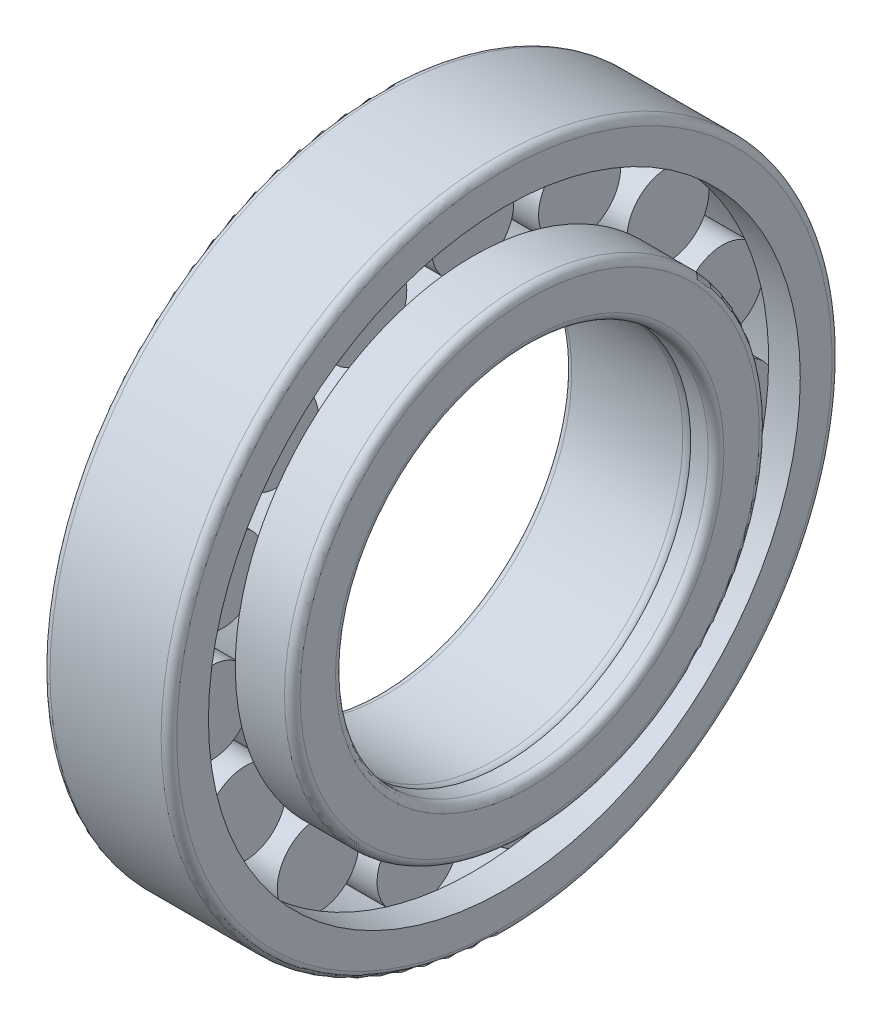
from build123d import *

# Parameters (mm, degrees)
SKETCH_3_W               = 17
SKETCH_3_H               = 11.0001
PATTERN_CIRCULAR_1_COUNT = 15


with BuildPart() as part:
    # 草图2 → Revolve 794 (revolve)
    with BuildSketch(Plane.XY, mode=Mode.PRIVATE) as revolve_794_sk:
        with BuildLine():
            Line((8.5, 59.5), (25.5, 59.5))
            Line((25.5, 59.5), (34, 57.222431864))
            Line((34, 57.222431864), (34, 52.1))
            ThreePointArc((34, 52.1), (33.38492424, 50.61507576), (31.9, 50))
            Line((31.9, 50), (2.1, 50))
            ThreePointArc((2.1, 50), (0.61507576, 50.61507576), (0, 52.1))
            Line((0, 52.1), (0, 63.7))
            Line((0, 63.7), (8.5, 63.7))
            Line((8.5, 63.7), (8.5, 59.5))
        make_face()
    revolve(revolve_794_sk.sketch.rotate(Axis((-10.080094127, 0, 0), (1, 0, 0)), 90), axis=Axis((-10.080094127, 0, 0), (1, 0, 0)))

    # 草图3 → 凸台-旋转1 (revolve)
    with BuildSketch(Plane.XY):
        with Locations((17, 64.99995)):
            Rectangle(SKETCH_3_W, SKETCH_3_H)
    revolve_1 = revolve(axis=Axis((-1.603948851, 70.5, 0), (1, 0, 0)))

    # 草图4 → 凸台-旋转2 (revolve)
    with BuildSketch(Plane.XY, mode=Mode.PRIVATE) as revolve_2_sk:
        with BuildLine():
            Line((25.5, 79.4), (34, 79.4))
            Line((34, 79.4), (34, 87.9))
            ThreePointArc((34, 87.9), (33.38492424, 89.38492424), (31.9, 90))
            Line((31.9, 90), (2.1, 90))
            ThreePointArc((2.1, 90), (0.61507576, 89.38492424), (0, 87.9))
            Line((0, 87.9), (0, 79.4))
            Line((0, 79.4), (8.5, 79.4))
            Line((8.5, 79.4), (8.5, 81.5))
            Line((8.5, 81.5), (25.5, 81.5))
            Line((25.5, 81.5), (25.5, 79.4))
        make_face()
    revolve(revolve_2_sk.sketch.rotate(Axis((0, 0, 0), (1, 0, 0)), 90), axis=Axis((0, 0, 0), (1, 0, 0)))

    # 草图5 → 凸台-旋转3 (revolve)
    with BuildSketch(Plane.XY, mode=Mode.PRIVATE) as revolve_3_sk:
        with BuildLine():
            Line((34, 57.222416261), (34, 50))
            Line((34, 50), (38.7, 50))
            ThreePointArc((38.7, 50), (40.18492424, 50.61507576), (40.8, 52.1))
            Line((40.8, 52.1), (40.8, 61.6))
            ThreePointArc((40.8, 61.6), (40.18492424, 63.08492424), (38.7, 63.7))
            Line((38.7, 63.7), (25.5, 63.7))
            Line((25.5, 63.7), (25.5, 59.499984397))
            Line((25.5, 59.499984397), (34, 57.222416261))
        make_face()
    revolve(revolve_3_sk.sketch.rotate(Axis((0, 0, 0), (1, 0, 0)), 90), axis=Axis((0, 0, 0), (1, 0, 0)))

    # 阵列(圆周)1: 凸台-旋转1 ×15 about axis
    pattern_circular_1_axis = Axis((0, 0, 0), (1, 0, 0))
    for i in range(1, PATTERN_CIRCULAR_1_COUNT):
        add(revolve_1.rotate(pattern_circular_1_axis, i * 360 / PATTERN_CIRCULAR_1_COUNT))


solid = part.part
